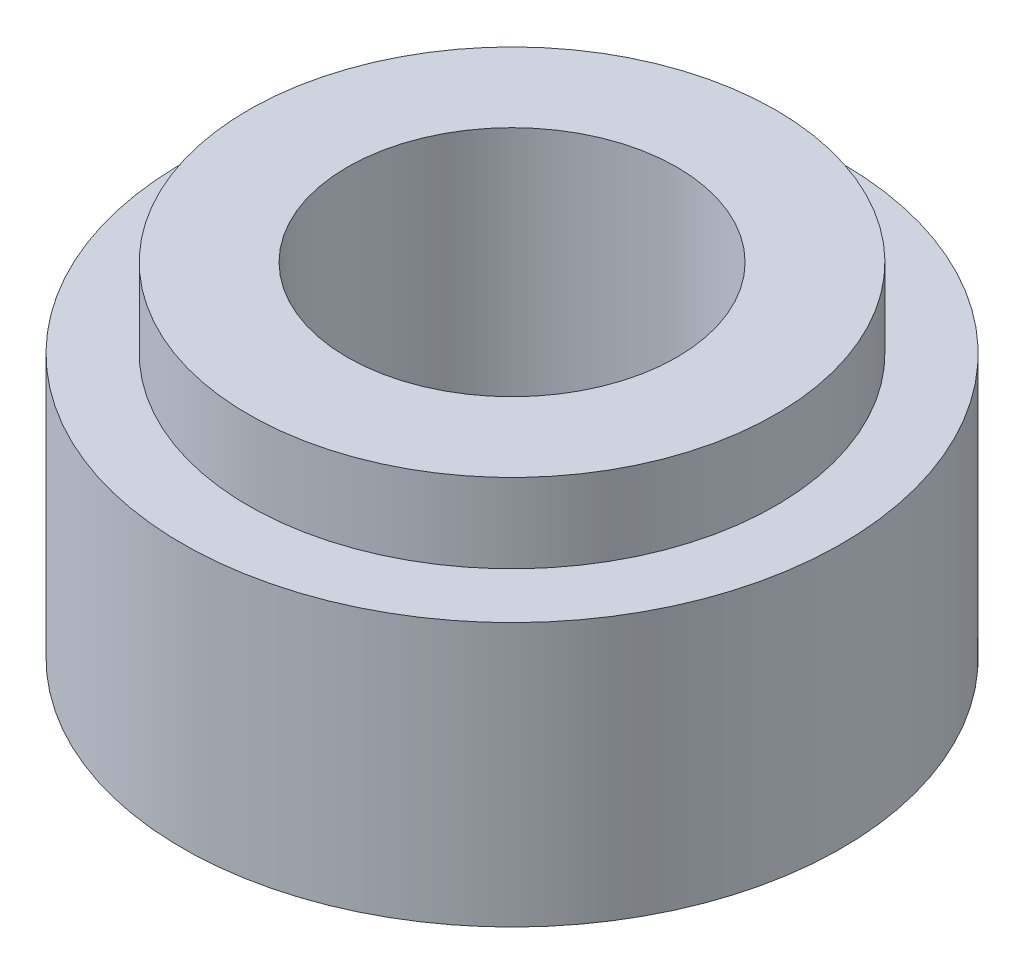
from build123d import *

# Parameters (mm, degrees)
M14X1_5_TAPPED_HOLE1_D     = 12.5
M14X1_5_TAPPED_HOLE1_DEPTH = 35.5
M14X1_5_TAPPED_HOLE1_TIP   = 3.755378869


with BuildPart() as part:
    # Sketch1 → Revolve1 (revolve)
    with BuildSketch(Plane.XY, mode=Mode.PRIVATE) as revolve1_sk:
        Polygon((0, 0), (12.5, 0), (12.5, 10), (10, 10), (10, 13), (0, 13), align=None)
    revolve(revolve1_sk.sketch.rotate(Axis((0, 0, 0), (0, 1, 0)), 90), axis=Axis((0, 0, 0), (0, 1, 0)))

    # M14x1.5 Tapped Hole1
    with Locations(Plane(origin=(0, 0, 0), x_dir=(-1, 0, 0), z_dir=(0, -1, 0))):
        with Locations((0, 0)):
            Hole(M14X1_5_TAPPED_HOLE1_D / 2, depth=M14X1_5_TAPPED_HOLE1_DEPTH)
            with Locations((0, 0, -(M14X1_5_TAPPED_HOLE1_DEPTH + M14X1_5_TAPPED_HOLE1_TIP / 2))):  # 118° drill point
                Cone(0, M14X1_5_TAPPED_HOLE1_D / 2, M14X1_5_TAPPED_HOLE1_TIP, mode=Mode.SUBTRACT)


solid = part.part
